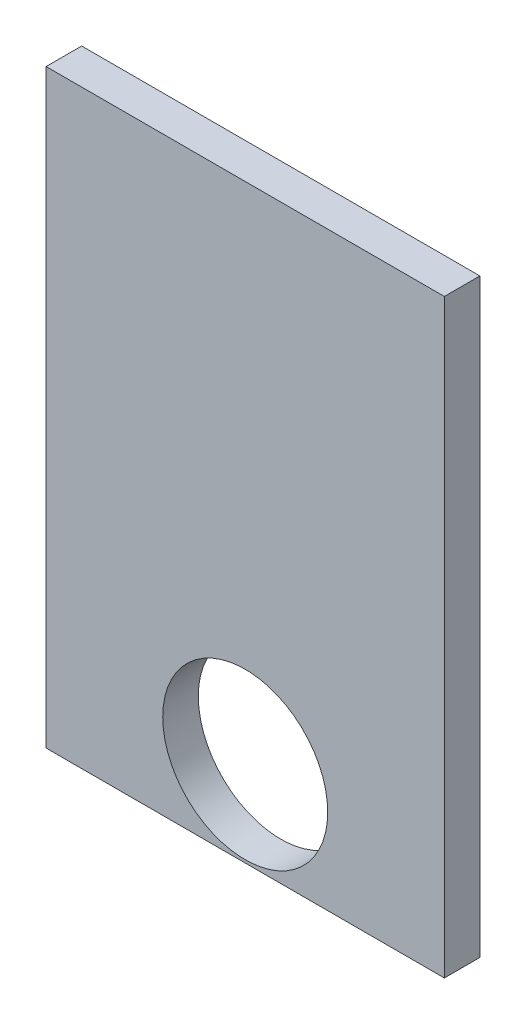
SolidWorks part; units mm, degrees
ref_plane "Front Plane" through (0, 0, 0) normal (0, 0, 1) x (1, 0, 0)
ref_plane "Top Plane" through (0, 0, 0) normal (0, 1, 0) x (1, 0, 0)
ref_plane "Right Plane" through (0, 0, 0) normal (1, 0, 0) x (0, 0, -1)
sketch "Sketch1" plane through (0, 0, 0) normal (0, 0, 1) x (1, 0, 0)
  line L1 (0, 0) -> (280, 0)
  line L2 (0, 0) -> (0, -415)
  line L3 (0, -415) -> (280, -415)
  line L4 (280, 0) -> (280, -415)
  circle A0 centre (140, -355) radius 58
  dimension "D3" = 116
  dimension "D1" = 280
  dimension "D2" = 415
extrude "Boss-Extrude1" add sketch "Sketch1" along normal blind 25
